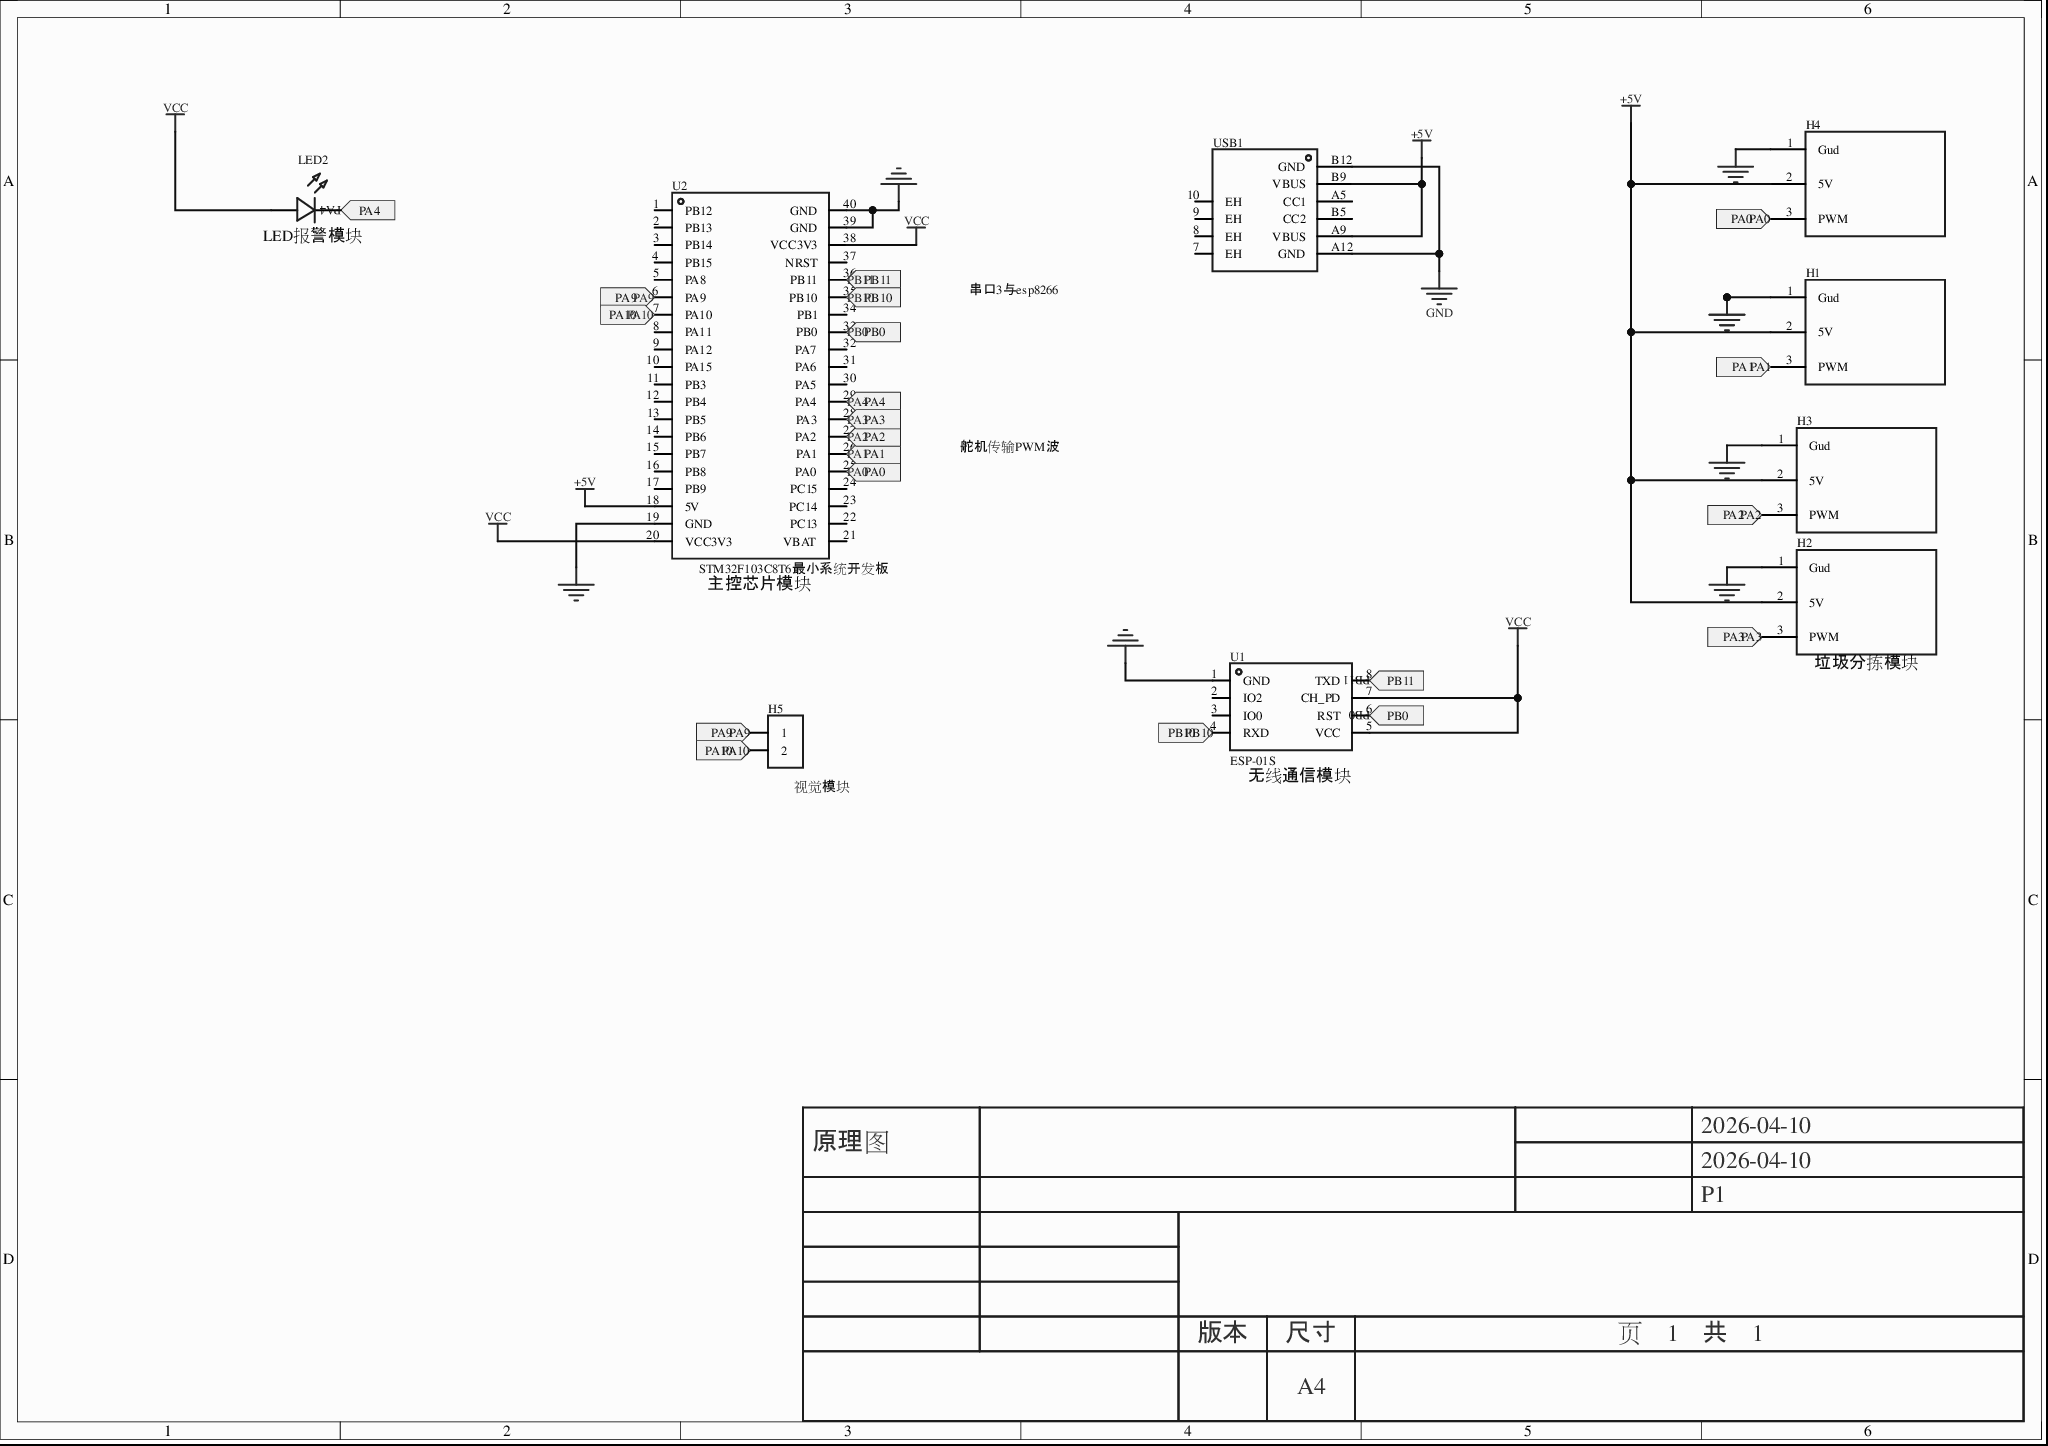
[diagram p0: MISC51955-3.schdoc]
# Altium project MISC51955-2.PrjPcb
1 sheet, 9 parts. Net scope: flat (ports and power ports of the same name join across sheets).
Board file: MISC51955.pcbdoc

## Sheet MISC51955-3.schdoc
size 297 x 209 mm; Version: V1.0; @Project Name: MISC51955; @Update Date: 2026-04-17; @Create Date: 2026-04-17; @Board Name: MISC51955; @Create Time: 18:08:13; @Page Count: 1; @Page No: 1; @Schematic Name: MISC51955; @Update Time: 18:08:13; Size: A4

### Parts
H1  (no value)  [HDR-TH_3P-P2.54-V-F]
H2  (no value)  [HDR-TH_3P-P2.54-V-F]
H3  (no value)  [HDR-TH_3P-P2.54-V-F]
H4  (no value)  [HDR-TH_3P-P2.54-V-F]
H5  (no value)  [HDR-TH_2P-P2.54-V-F]
LED2  (no value)  [LED_TH-3mm]
U1  ESP-01S  [WIFIM-TH_ESP-01S]
U2  STM32F103C8T6最小系统开发板  [CONN-TH_L53.3-W22.9_STM32F103C8T6-CARD]
USB1  (no value)  [USB_ TYPE-C-6P]

### Ports
PA0 (in), PA1 (in), PA2 (in), PA3 (in), PA4 (in), PA9 (in), PA10 (in), PB0 (in), PB10 (in), PB11 (in)

### Nets
+5V: H1.2(5V) H2.2(5V) H3.2(5V) H4.2(5V) U2.18(5V) USB1.A9(VBUS) USB1.B9(VBUS)
GND: H1.1(Gud) H2.1(Gud) H3.1(Gud) H4.1(Gud) U1.1(GND) U2.19(GND) U2.39(GND) U2.40(GND) USB1.A12(GND) USB1.B12(GND)
VCC: LED2.1(C) U1.5(VCC) U1.7(CH_PD) U2.20(VCC3V3) U2.38(VCC3V3)
PA0: H4.3(PWM) U2.25(PA0) ; port PA0
PA1: H1.3(PWM) U2.26(PA1) ; port PA1
PA2: H3.3(PWM) U2.27(PA2) ; port PA2
PA3: H2.3(PWM) U2.28(PA3) ; port PA3
PA4: LED2.2(A) U2.29(PA4) ; port PA4
PA9: H5.1 U2.6(PA9) ; port PA9
PA10: H5.2 U2.7(PA10) ; port PA10
PB0: U1.6(RST) U2.33(PB0) ; port PB0
PB10: U1.4(RXD) U2.35(PB10) ; port PB10
PB11: U1.8(TXD) U2.36(PB11) ; port PB11

Not connected (* = marked no-connect by the designer): U1 2(IO2)* 3(IO0)*; U2 1(PB12)* 2(PB13)* 3(PB14)* 4(PB15)* 5(PA8)* 8(PA11)* 9(PA12)* 10(PA15)* 11(PB3)* 12(PB4)* 13(PB5)* 14(PB6)* 15(PB7)* 16(PB8)* 17(PB9)* 21(VBAT)* 22(PC13)* 23(PC14)* 24(PC15)* 30(PA5)* 31(PA6)* 32(PA7)* 34(PB1)* 37(NRST)*; USB1 7(EH) 8(EH) 9(EH) 10(EH) A5(CC1) B5(CC2)

### Notes on the sheet
- (near LED2) LED报警模块
- 串口3与esp8266
- 舵机传输PWM波
- (near U2) 主控芯片模块
- (near H2) 垃圾分拣模块
- (near U1) 无线通信模块
- (near H5) 视觉模块
- 2026-04-10
- 原理图
- P1
- 版本
- 尺寸
- A4
- 页    1    共    1

### Library data of the parts
H1-H4 = GS90: AddInBom: yes; Device: GS90; Symbol: GS90; ConvertToPcb: yes
H5 = HDR-F_2.54_1x2P: Symbol: Header-Female-2.54_1x2; ConvertToPcb: yes; ModelId: a9450ef445564560a104363b9aacde4e0819f05c4eef4c71ace90d822a990e87; ModelName: HDR-TH_2P-P2.54-F-LI-1X2P; ModelTransform: 215.7476,98.425,0,0,0,0,0,0,-129.921; Device: HDR-F_2.54_1x2P; AddInBom: yes; SupplierPart: C49661; Supplier Footprint: 插件; FootprintName: HDR-TH_2P-P2.54-V-F
LED2 = LED_TH-R_3mm: ConvertToPcb: yes; ModelId: a497c992633541038a38947cdc58012f0819f05c4eef4c71ace90d822a990e87; ModelName: LED-TH-3mm_R; ModelTransform: 141.274,153.327,0,0,0,0,-5.984,0,-137.795; Device: LED_TH-R_3mm; Symbol: LED_TH-R; FootprintName: LED_TH-3mm; AddInBom: yes; Supplier Footprint: 插件
U1 = ESP-01S_C111009: AddInBom: yes; ModelId: eb7175da78ae48b3b1568cfe3027405f0819f05c4eef4c71ace90d822a990e87; ModelTransform: 582.676,976.37608,0,0,0,0,0,388.346,-118.11; Device: ESP-01S_C111009; Symbol: ESP-01S; FootprintName: WIFIM-TH_ESP-01S; LCSC Part Name: ESP-01S; SupplierPart: C111009; ManufacturerPart: ESP-01S; Supplier Footprint: -; JLCPCB Part Class: Extended Part; Supplier: LCSC; ConvertToPcb: yes; ModelName: WIFIM-TH_ESP-01S
U2 = STM32F103C8T6-Card: AddInBom: yes; ModelId: 12c257eccf3b4e5baa9346e6693d8ea4; Device: STM32F103C8T6-Card; Symbol: STM32F103C8T6-CARD; Manufacturer Part: STM32F103C8T6最小系统开发板; FootprintName: CONN-TH_L53.3-W22.9_STM32F103C8T6-CARD; LCSC Part Name: STM32F103C8T6-Card; SupplierPart: C9900077949; Supplier Footprint: 插件; JLCPCB Part Class: Extended Part; Supplier: LCSC; ConvertToPcb: yes; ModelName: CONN-TH_L53.3-W22.9_STM32F103C8T6-CARD
USB1 = USB_ Type-C-6P: AddInBom: yes; ModelId: d4f492a4e6024845a13b3f6a4ef2d2cb0819f05c4eef4c71ace90d822a990e87; ModelName: USB-SMD_U262-061N-4BVC11; ModelTransform: 352.362,281.496,0,0,0,0,0,-47.244,-39.37; Device: USB_ Type-C-6P; Symbol: USB_ TYPE-C-6P; FootprintName: USB_ TYPE-C-6P; Supplier Footprint: SMD; ConvertToPcb: yes